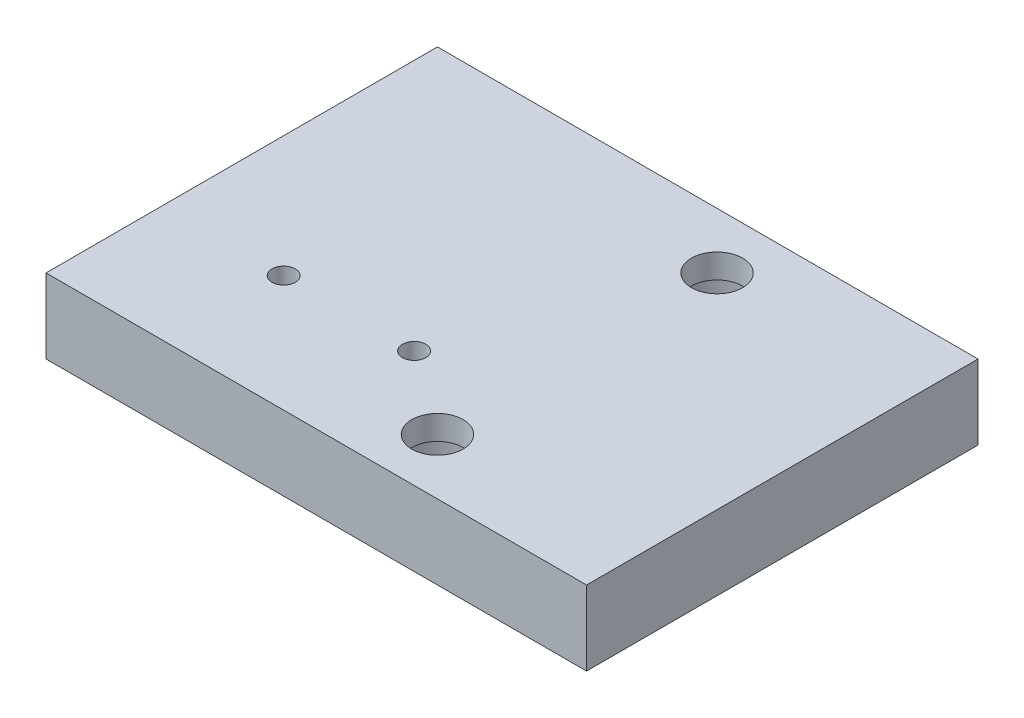
SolidWorks part; units mm, degrees
material "AL6061"
ref_plane "前视基准面" through (0, 0, 0) normal (0, 0, 1) x (1, 0, 0)
ref_plane "上视基准面" through (0, 0, 0) normal (0, 1, 0) x (1, 0, 0)
ref_plane "右视基准面" through (0, 0, 0) normal (1, 0, 0) x (0, 0, -1)
sketch "草图1" plane through (0, 0, 0) normal (0, 1, 0) x (1, 0, 0)
  line L1 (-29, 21) -> (29, 21)
  line L2 (-29, 21) -> (-29, -21)
  line L3 (-29, -21) -> (29, -21)
  line L4 (29, 21) -> (29, -21)
  line L5 (-29, 21) -> (29, -21) construction
  line L6 (-29, -21) -> (29, 21) construction
  point P0 (0, 0)
  dimension "D1" = 42
  dimension "D2" = 58
extrude "凸台-拉伸1" add sketch "草图1" along normal mid plane 8
sketch "草图2" plane through (0, -4, 0) normal (0, -1, 0) x (-1, 0, 0)
  point P0 (-7, 15)
  point P3 (-7, -15)
hole_wizard "M5 六角凹头螺钉的柱形沉头孔1" positions "草图2" profile "草图3" counterbore size "M5" standard "ISO" end condition through all
sketch "草图3" plane through (7, -4, -15) normal (1, 0, 0) x (0, 0, -1)
  line L0 (0, 0) -> (0, 8)
  line L1 (0, 8) -> (2.75, 8)
  line L3 (2.75, 8) -> (2.75, 5.4)
  line L4 (2.75, 5.4) -> (5, 5.4)
  line L5 (5, 5.4) -> (5, 0)
  line L7 (5, 0) -> (0, 0)
  line L11 (0, -6.35) -> (0, 107.95) construction
  dimension "通孔孔直径" = 5.5
  dimension "通孔孔深度" = 8
  dimension "柱形沉头孔直径" = 10
  dimension "柱形沉头孔深度" = 5.4
sketch "草图4" plane through (-29, 0, 0) normal (-1, 0, 0) x (0, 0, 1)
  line L0 (0, 0) -> (0, 6.8721) construction
  line L1 (-21, 4) -> (-21, -4) construction
  point P0 (-11, 0)
  point P9 (11, 0)
  dimension "D1" = 10
hole_wizard "M4 螺纹孔1" positions "草图4" profile "草图5" tap size "M4" standard "ISO"
sketch "草图5" plane through (-29, 0, -11) normal (0, 1, 0) x (0, 0, 1)
  line L0 (0, 0) -> (0, 11.0914)
  line L1 (0, 11.0914) -> (1.65, 10.1)
  line L2 (1.65, 10.1) -> (1.65, 0)
  line L5 (1.65, 0) -> (0, 0)
  line L10 (0, 11.0914) -> (-1.65, 10.1) construction
  line L11 (0, -6.35) -> (0, 107.95) construction
  dimension "螺纹孔钻头直径" = 3.3
  dimension "螺纹孔钻头深度" = 10.1
  dimension "导头角度" = 118
cosmetic thread "孔螺蚊线1" parameters "D1"=8, "D2"=4
cosmetic thread "孔螺蚊线2" parameters "D1"=8, "D2"=4
sketch "草图6" plane through (0, -4, 0) normal (0, -1, 0) x (-1, 0, 0)
  point P0 (16, -8.5)
  point P3 (2, -8.5)
hole_wizard "M3 螺纹孔1" positions "草图6" profile "草图7" tap size "M3" standard "GB" end condition through all
sketch "草图7" plane through (-16, -4, 8.5) normal (1, 0, 0) x (0, 0, -1)
  line L0 (0, 0) -> (0, 8)
  line L1 (0, 8) -> (1.25, 8)
  line L2 (1.25, 8) -> (1.25, 0)
  line L5 (1.25, 0) -> (0, 0)
  line L11 (0, -6.35) -> (0, 107.95) construction
  dimension "通孔螺纹孔钻头直径" = 2.5
  dimension "通孔螺纹孔钻头深度" = 8
cosmetic thread "孔螺蚊线3" parameters "D2"=3
cosmetic thread "孔螺蚊线4" parameters "D2"=3
